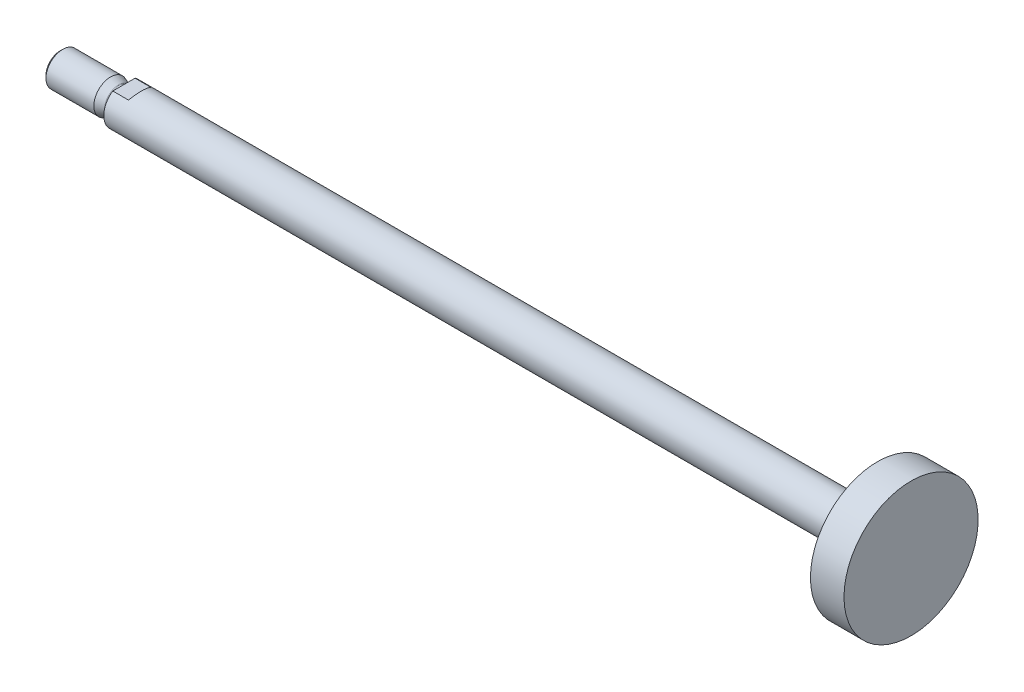
from build123d import *

# Parameters (mm, degrees)
SKETCH_1_W          = 10
SKETCH_1_H          = 20
SKETCH_2_R          = 6
EXTRUDE_1_DEPTH     = 224.7
CUT_EXTRUDE_START   = -4.7
CUT_EXTRUDE_1_DEPTH = 4.7
CUT_EXTRUDE_2_DEPTH = 4.7
SKETCH_5_R          = 4.1
EXTRUDE_2_DEPTH     = 1.5
SKETCH_6_R          = 4.1
EXTRUDE_3_DEPTH     = 2.472729678
EXTRUDE_3_DRAFT     = -20
SKETCH_7_R          = 5
EXTRUDE_4_DEPTH     = 15.027270322
DRAFT_1_ANGLE       = 30
DRAFT_2_ANGLE       = 30
CHAMFER_1_SIZE      = 0.767
FILLET_1_R          = 0.6


with BuildPart() as part:
    # 草图1 → 旋转1 (revolve)
    with BuildSketch(Plane(origin=(0, 0, 0), x_dir=(-1, 0, 0), z_dir=(0, 0, -1)), mode=Mode.PRIVATE) as revolve_1_sk:
        with Locations((-223.6, 10)):
            Rectangle(SKETCH_1_W, SKETCH_1_H)
    revolve(revolve_1_sk.sketch.rotate(Axis((228.6, 0, 0), (-1, 0, 0)), 270), axis=Axis((228.6, 0, 0), (-1, 0, 0)))

    # 草图2 → 凸台-拉伸1 (add)
    with BuildSketch(Plane.ZY.offset(-218.6)):
        Circle(SKETCH_2_R)
    extrude(amount=EXTRUDE_1_DEPTH)

    # 草图3 → 切除-拉伸1 (cut)
    with BuildSketch(Plane.ZY.offset(6.1).offset(CUT_EXTRUDE_START)):
        with BuildLine():
            Line((-3.31662479, 5), (3.31662479, 5))
            ThreePointArc((3.31662479, 5), (0, 6), (-3.31662479, 5))
        make_face()
    extrude(amount=CUT_EXTRUDE_1_DEPTH, mode=Mode.SUBTRACT)

    # 草图4 → 切除-拉伸2 (cut)
    with BuildSketch(Plane.ZY.offset(6.1).offset(CUT_EXTRUDE_START)):
        with BuildLine():
            Line((3.31662479, -5), (-3.31662479, -5))
            ThreePointArc((-3.31662479, -5), (0, -6), (3.31662479, -5))
        make_face()
    extrude(amount=CUT_EXTRUDE_2_DEPTH, mode=Mode.SUBTRACT)

    # 草图5 → 凸台-拉伸2 (add)
    with BuildSketch(Plane.ZY.offset(6.1)):
        Circle(SKETCH_5_R)
    extrude(amount=EXTRUDE_2_DEPTH)


with BuildPart() as extrude_3_tool:
    # 草图6 → 凸台-拉伸3 (with draft: the straight prism first)
    with BuildSketch(Plane.ZY.offset(7.6)):
        Circle(SKETCH_6_R)
    extrude(amount=EXTRUDE_3_DEPTH)
    # 凸台-拉伸3: the draft: its side faces are tilted about the plane it starts from
    extrude_3_sides = [extrude_3_tool.faces().sort_by_distance(p)[0] for p in [
        (-8.836364839, 0, -4.1),
    ]]
    draft(extrude_3_sides, Plane.ZY.offset(7.6), EXTRUDE_3_DRAFT)


with BuildPart() as part_1:
    add(part.part)

    # 凸台-拉伸3: add extrude_3_tool
    add(extrude_3_tool.part)

    # 草图7 → 凸台-拉伸4 (add)
    with BuildSketch(Plane.ZY.offset(10.072729678)):
        with Locations(Location((0, 0, 0), (0, 0, 180))):
            Circle(SKETCH_7_R)
    extrude(amount=EXTRUDE_4_DEPTH)

    # 拔模1
    draft_1_faces = [part_1.faces().sort_by_distance(p)[0] for p in [
        (-1.4, -5.403002256, 0),
    ]]
    draft(draft_1_faces, Plane(origin=(-1.4, -5, 3.31662479), x_dir=(0, 0, -1), z_dir=(0, -1, 0)), DRAFT_1_ANGLE)

    # 拔模2
    draft_2_faces = [part_1.faces().sort_by_distance(p)[0] for p in [
        (-1.4, 5.403002256, 0),
    ]]
    draft(draft_2_faces, Plane(origin=(-1.4, 5, -3.31662479), x_dir=(0, 0, 1), z_dir=(0, 1, 0)), DRAFT_2_ANGLE)

    # 倒角1
    chamfer_1_edges = [part_1.edges().sort_by_distance(p)[0] for p in [
        (-25.1, 0, 5),
    ]]
    chamfer(chamfer_1_edges, length=CHAMFER_1_SIZE)

    # 圆角1
    fillet_1_edges = [part_1.edges().sort_by_distance(p)[0] for p in [
        (-6.1, 0, -4.1),
        (-7.6, 0, -4.1),
    ]]
    fillet(fillet_1_edges, radius=FILLET_1_R)


solid = part_1.part
